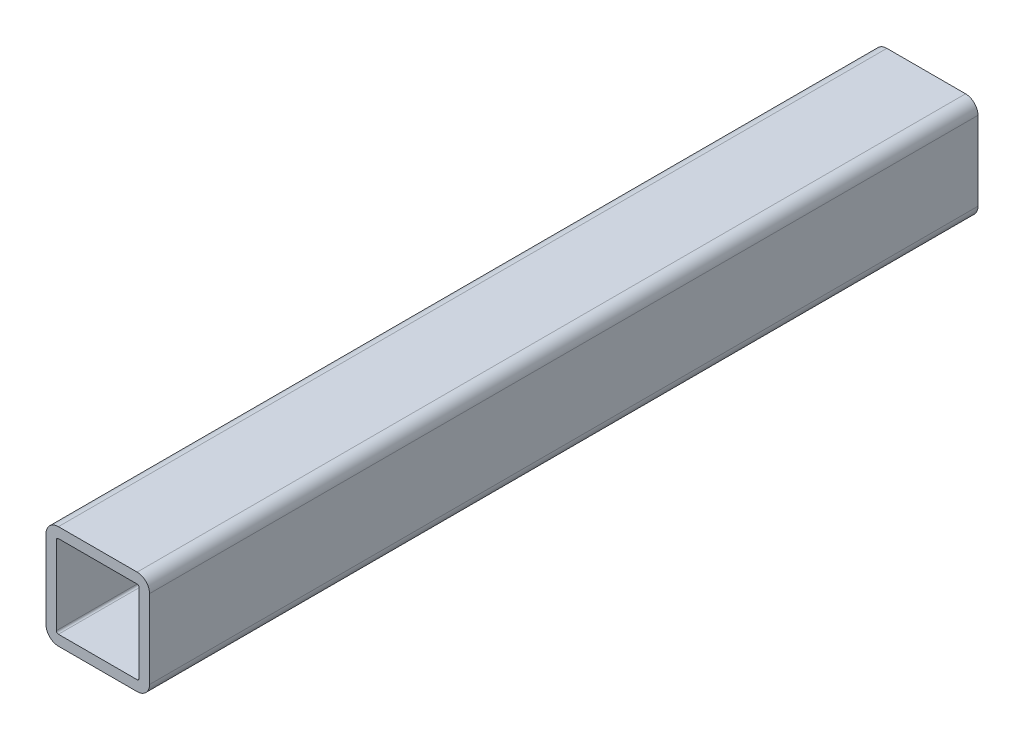
from build123d import *

# Parameters (mm, degrees)
BOSS_EXTRUDE1_DEPTH = 400


with BuildPart() as part:
    # Sketch1 → Boss-Extrude1 (new body)
    with BuildSketch(Plane.XY):
        with BuildLine():
            Line((6, 0), (44, 0))
            ThreePointArc((44, 0), (48.242640687, 1.757359313), (50, 6))
            Line((50, 6), (50, 44))
            ThreePointArc((50, 44), (48.242640687, 48.242640687), (44, 50))
            Line((44, 50), (6, 50))
            ThreePointArc((6, 50), (1.757359313, 48.242640687), (0, 44))
            Line((0, 44), (0, 6))
            ThreePointArc((0, 6), (1.757359313, 1.757359313), (6, 0))
        make_face()
        with BuildLine():
            Line((6, 45), (44, 45))
            ThreePointArc((44, 45), (44.707106781, 44.707106781), (45, 44))
            Line((45, 44), (45, 6))
            ThreePointArc((45, 6), (44.707106781, 5.292893219), (44, 5))
            Line((44, 5), (6, 5))
            ThreePointArc((6, 5), (5.292893219, 5.292893219), (5, 6))
            Line((5, 6), (5, 44))
            ThreePointArc((5, 44), (5.292893219, 44.707106781), (6, 45))
        make_face(mode=Mode.SUBTRACT)
    extrude(amount=BOSS_EXTRUDE1_DEPTH)


solid = part.part
